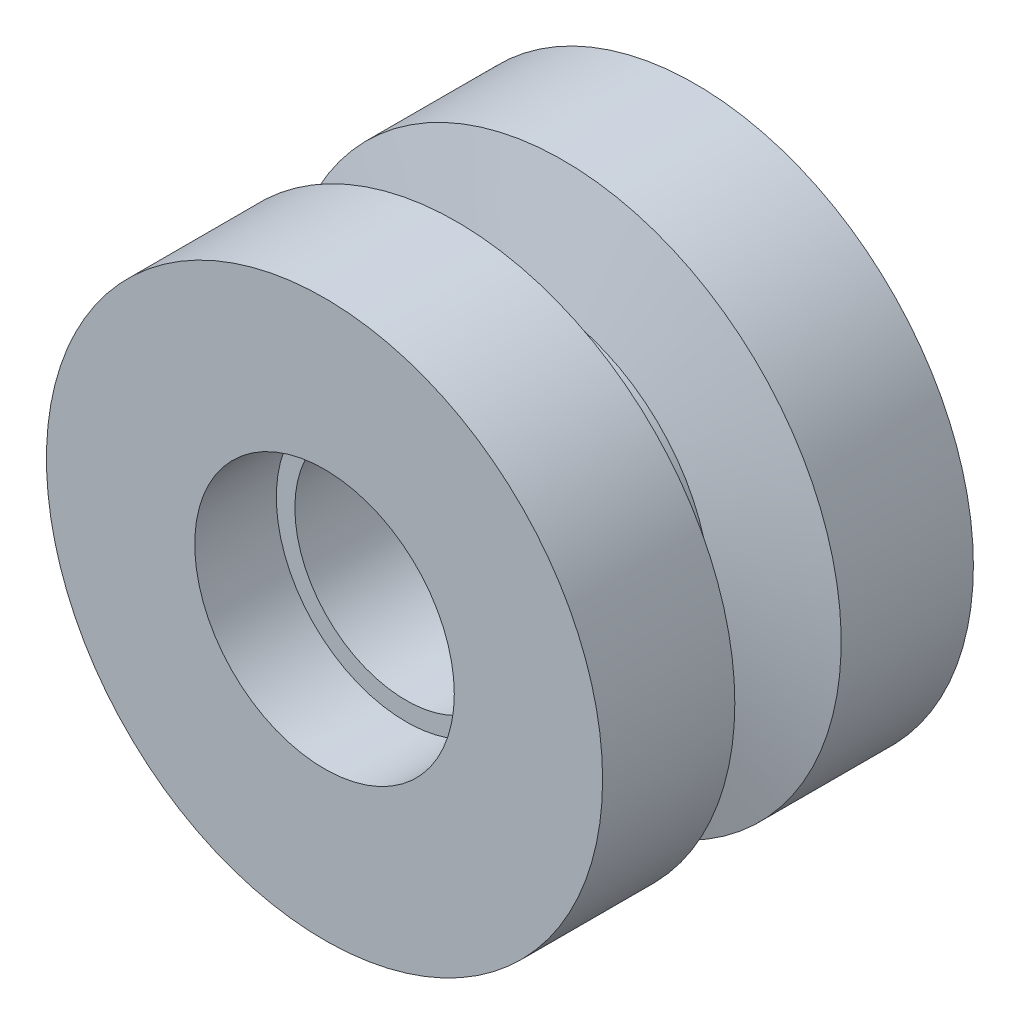
SolidWorks part; units mm, degrees
material "普通碳钢"
ref_plane "前视基准面" through (0, 0, 0) normal (0, 0, 1) x (1, 0, 0)
ref_plane "上视基准面" through (0, 0, 0) normal (0, 1, 0) x (1, 0, 0)
ref_plane "右视基准面" through (0, 0, 0) normal (1, 0, 0) x (0, 0, -1)
sketch "草图1" plane through (0, 0, 0) normal (0, 0, 1) x (1, 0, 0)
  circle A0 centre (0, 0) radius 37.5
  circle A1 centre (0, 0) radius 15
  dimension "D1" = 75
  dimension "D2" = 30
extrude "凸台-拉伸1" add sketch "草图1" along normal blind 50
sketch "草图2" plane through (0, 0, 0) normal (0, 1, 0) x (1, 0, 0)
  line L0 (37.5, -25) -> (-44.7851, -25) construction
  line L1 (37.5, -50) -> (37.5, 0) construction
  line L2 (0, 0) -> (0, -52.3687) construction
  line L3 (-38.25, -17.6488) -> (-23.25, -21.25)
  line L4 (-23.25, -21.25) -> (-23.25, -28.75)
  line L5 (-38.25, -17.6488) -> (-38.25, -32.3512)
  line L6 (-38.25, -32.3512) -> (-23.25, -28.75)
  point P11 (-23.25, -25)
  point P13 (-38.25, -25)
  dimension "D1" = 23.25
  dimension "D2" = 3.75
  dimension "D3" = 13.5
  dimension "D4" = 15
revolve "切除-旋转1" cut sketch "草图2" angle 360 about L2
sketch "草图3" plane through (0, 0, 50) normal (0, 0, 1) x (1, 0, 0)
  circle A0 centre (0, 0) radius 17.5
  dimension "D1" = 35
extrude "切除-拉伸1" cut sketch "草图3" against normal blind 11
sketch "草图4" plane through (0, 0, 0) normal (0, 0, -1) x (-1, 0, 0)
  circle A0 centre (0, 0) radius 17.5
  dimension "D1" = 35
extrude "切除-拉伸2" cut sketch "草图4" against normal blind 11
